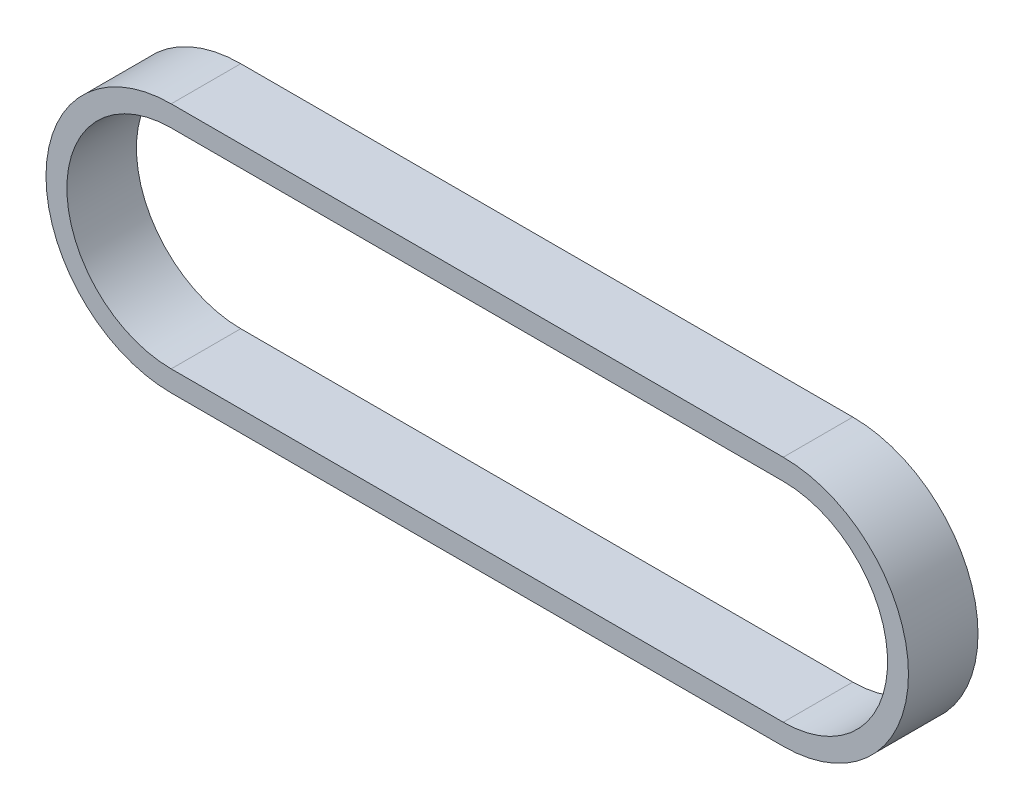
SolidWorks part; units mm, degrees
ref_plane "Front Plane" through (0, 0, 0) normal (0, 0, 1) x (1, 0, 0)
ref_plane "Top Plane" through (0, 0, 0) normal (0, 1, 0) x (1, 0, 0)
ref_plane "Right Plane" through (0, 0, 0) normal (1, 0, 0) x (0, 0, -1)
sketch "Sketch2" plane through (0, 0, 0) normal (0, 0, 1) x (1, 0, 0)
  line L0 (55, 0) -> (-55, 0) construction
  line L1 (0, 18) -> (-88, 18)
  line L2 (0, -18) -> (-88, -18)
  arc A0 (0, -18) -> (0, 18) centre (0, 0) ccw
  arc A1 (-88, 18) -> (-88, -18) centre (-88, 0) ccw
  dimension "D1" = 36
  dimension "D2" = 36
  dimension "D3" = 88
extrude "Boss-Extrude1" add sketch "Sketch2" along normal blind 10
shell "Shell1" thickness 3
